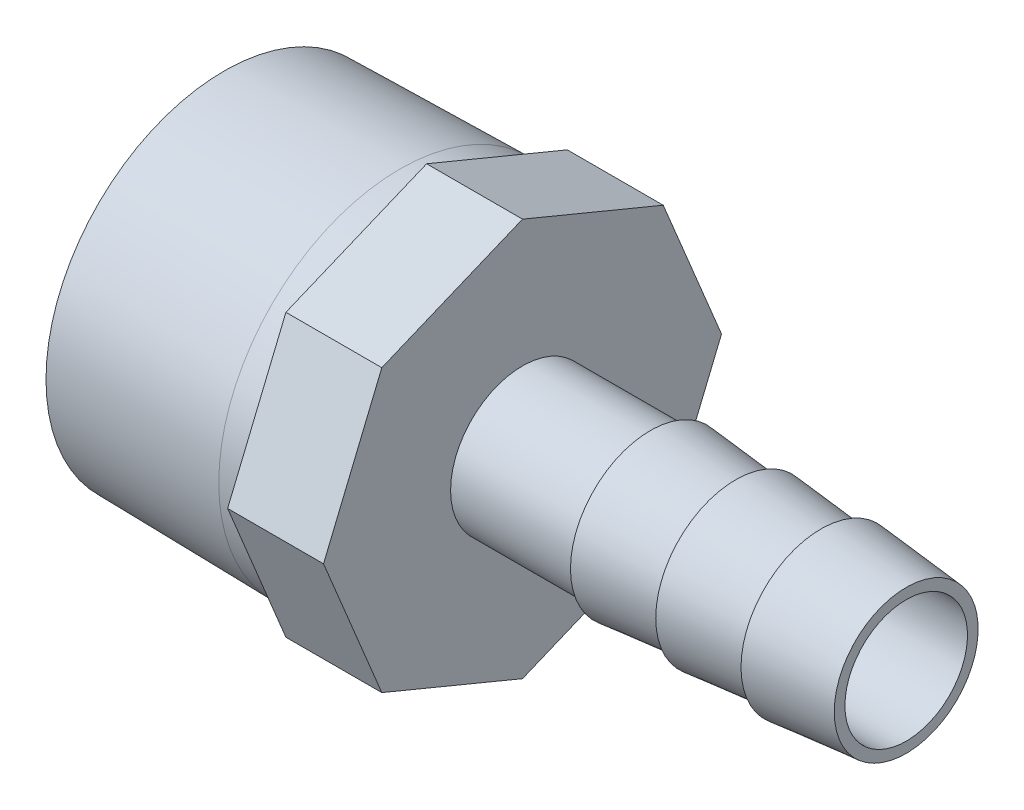
from build123d import *

# Parameters (mm, degrees)
SKETCH4_R           = 17
BOSS_EXTRUDE1_DEPTH = 9


with BuildPart() as part:
    # Sketch1 → Revolve1 (revolve)
    with BuildSketch(Plane.XY, mode=Mode.PRIVATE) as revolve1_sk:
        Polygon((19, 17), (19, 17.25), (28, 17.25), (28, 6.75), (40, 6.75), (40, 7.5), (48, 6.75), (48, 7.5), (56, 6.75), (56, 7.5), (64, 6.75), (64, 5.75), (26, 5.75), (26, 14), (0, 14), (0, 16.711991429), (16.5, 17), align=None)
    revolve(revolve1_sk.sketch.rotate(Axis((0, 0, 0), (1, 0, 0)), 90), axis=Axis((0, 0, 0), (1, 0, 0)))

    # Sketch4 → Boss-Extrude1 (add)
    with BuildSketch(Plane(origin=(28, 0, 0), x_dir=(0, 0, -1), z_dir=(1, 0, 0))):
        Polygon((0, 18.671265455), (-13.202578417, 13.202578417), (-18.671265455, 0), (-13.202578417, -13.202578417), (0, -18.671265455), (13.202578417, -13.202578417), (18.671265455, 0), (13.202578417, 13.202578417), align=None)
        with Locations(Location((0, 0, 0), (0, 0, 180))):
            Circle(SKETCH4_R, mode=Mode.SUBTRACT)
    extrude(amount=-BOSS_EXTRUDE1_DEPTH)


solid = part.part
